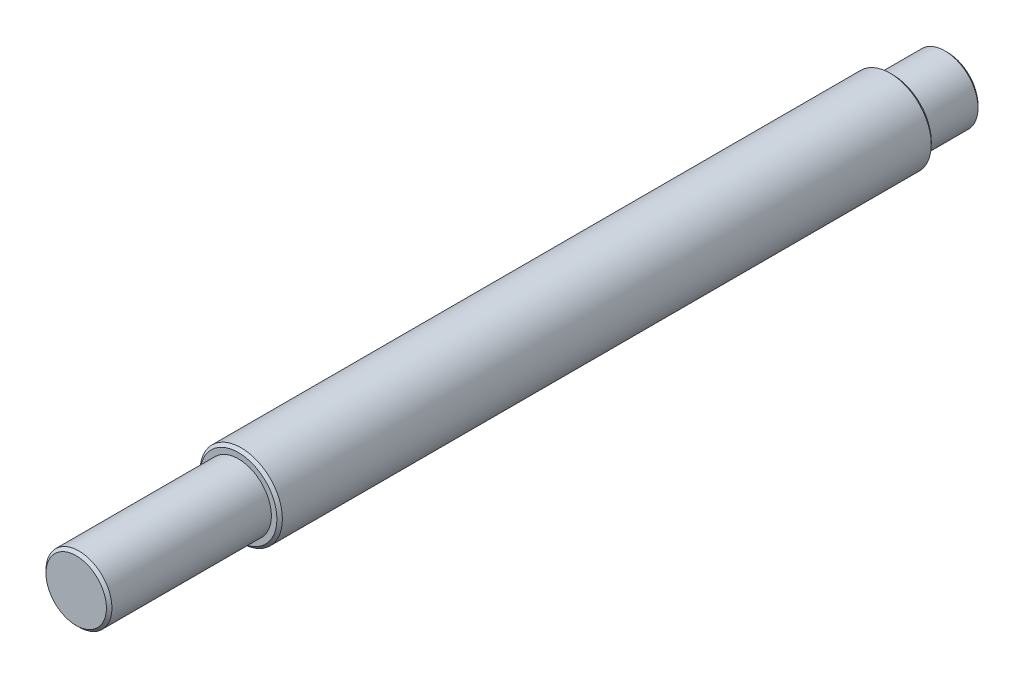
from build123d import *

# Parameters (mm, degrees)
SKETCH_1_R          = 7.5
EXTRUDE_1_DEPTH     = 158.5
SKETCH_5_OUTSIDE_W  = 48.982
SKETCH_5_OUTSIDE_H  = 48.982
SKETCH_5_OUTSIDE_R  = 6
CUT_EXTRUDE_3_DEPTH = 29.5
CHAMFER_2_SIZE      = 0.5
SKETCH_2_OUTSIDE_W  = 48.982
SKETCH_2_OUTSIDE_H  = 48.982
SKETCH_2_OUTSIDE_R  = 6
CUT_EXTRUDE_4_DEPTH = 10
CHAMFER_3_SIZE      = 0.5
CUT_EXTRUDE_START   = -4
CUT_EXTRUDE_5_DEPTH = 48


with BuildPart() as part:
    # 草图1 → 凸台-拉伸1 (new body)
    with BuildSketch(Plane.XY):
        Circle(SKETCH_1_R)
    extrude(amount=-EXTRUDE_1_DEPTH)

    # 草图5 outside → 切除-拉伸3 (cut)
    with BuildSketch(Plane.XY):
        Rectangle(SKETCH_5_OUTSIDE_W, SKETCH_5_OUTSIDE_H)
        Circle(SKETCH_5_OUTSIDE_R, mode=Mode.SUBTRACT)
    extrude(amount=-CUT_EXTRUDE_3_DEPTH, mode=Mode.SUBTRACT)

    # 倒角2
    chamfer_2_edges = [part.edges().sort_by_distance(p)[0] for p in [
        (-7.5, 0, -29.5),
        (-6, 0, 0),
    ]]
    chamfer(chamfer_2_edges, length=CHAMFER_2_SIZE)

    # 草图2 outside → 切除-拉伸4 (cut)
    with BuildSketch(Plane(origin=(0, 0, -158.5), x_dir=(-1, 0, 0), z_dir=(0, 0, -1))):
        Rectangle(SKETCH_2_OUTSIDE_W, SKETCH_2_OUTSIDE_H)
        with Locations(Location((0, 0, 0), (0, 0, 180))):
            Circle(SKETCH_2_OUTSIDE_R, mode=Mode.SUBTRACT)
    extrude(amount=-CUT_EXTRUDE_4_DEPTH, mode=Mode.SUBTRACT)

    # 倒角3
    chamfer_3_edges = [part.edges().sort_by_distance(p)[0] for p in [
        (-7.5, 0, -148.5),
        (-6, 0, -158.5),
    ]]
    chamfer(chamfer_3_edges, length=CHAMFER_3_SIZE)

    # 草图8 → 切除-拉伸5 (cut)
    with BuildSketch(Plane(origin=(0, 0, 0), x_dir=(1, 0, 0), z_dir=(0, 1, 0)).offset(CUT_EXTRUDE_START)):
        with BuildLine():
            Line((2.5, 57.5), (2.5, 32.5))
            ThreePointArc((2.5, 32.5), (0, 30), (-2.5, 32.5))
            Line((-2.5, 32.5), (-2.5, 57.5))
            ThreePointArc((-2.5, 57.5), (0, 60), (2.5, 57.5))
        make_face()
        with BuildLine():
            Line((2.5, 145.5), (2.5, 120.5))
            ThreePointArc((2.5, 120.5), (0, 118), (-2.5, 120.5))
            Line((-2.5, 120.5), (-2.5, 145.5))
            ThreePointArc((-2.5, 145.5), (0, 148), (2.5, 145.5))
        make_face()
    extrude(amount=-CUT_EXTRUDE_5_DEPTH, mode=Mode.SUBTRACT)


solid = part.part
